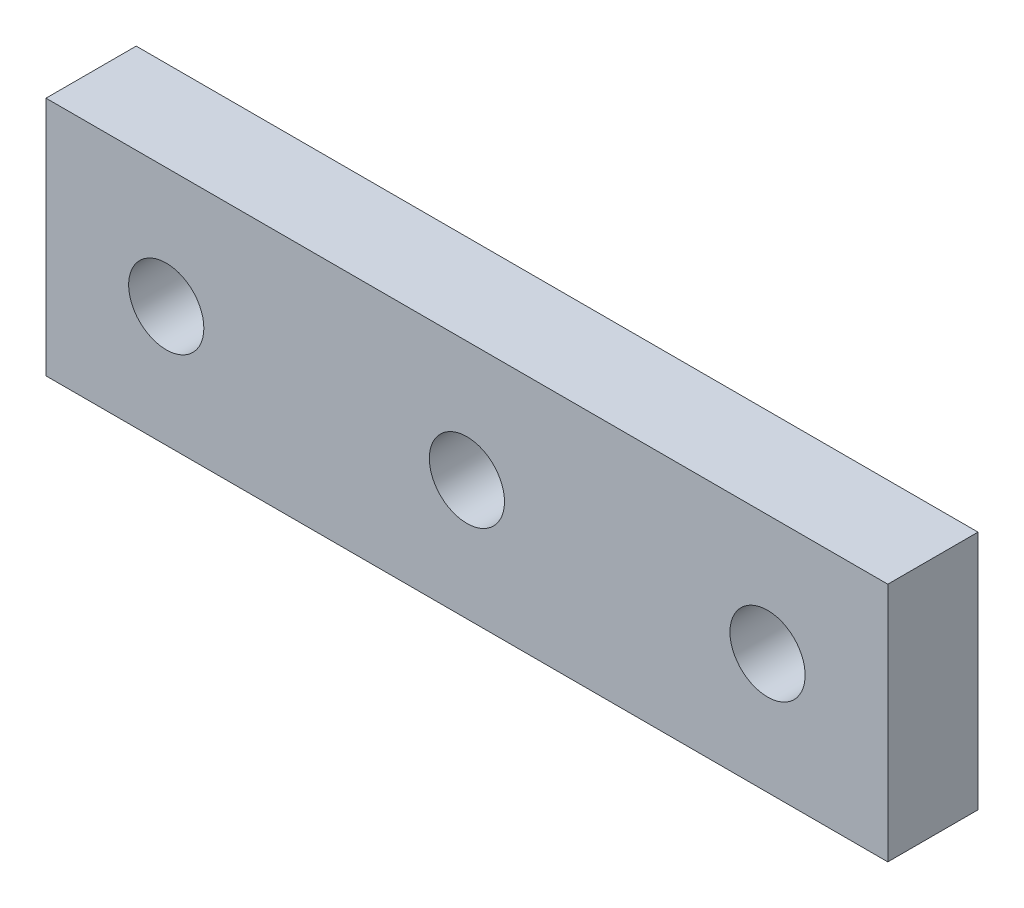
from build123d import *

# Parameters (mm, degrees)
SKETCH1_W             = 28
SKETCH1_H             = 8
SKETCH1_R             = 1.25
BOSS_EXTRUDE1_DEPTH   = 3
M3_TAPPED_HOLE6_D     = 2.5
M3_TAPPED_HOLE6_DEPTH = 7.5
M3_TAPPED_HOLE6_TIP   = 0.751075774
M3_TAPPED_HOLE1_D     = 2.5
M3_TAPPED_HOLE1_DEPTH = 7.5
M3_TAPPED_HOLE1_TIP   = 0.751075774


with BuildPart() as part:
    # Sketch1 → Boss-Extrude1 (new body)
    with BuildSketch(Plane.XY):
        with Locations((14, -4)):
            Rectangle(SKETCH1_W, SKETCH1_H)
        with Locations((4, -4)):
            Circle(SKETCH1_R, mode=Mode.SUBTRACT)
        with Locations(Location((24, -4, 0), (0, 0, 180))):
            Circle(SKETCH1_R, mode=Mode.SUBTRACT)
    extrude(amount=BOSS_EXTRUDE1_DEPTH)

    # M3 Tapped Hole6
    with Locations(Plane(origin=(4, -4, 3), x_dir=(1, 0, 0), z_dir=(0, 0, 1))):
        with Locations((0, 0), (20, 0)):
            Hole(M3_TAPPED_HOLE6_D / 2, depth=M3_TAPPED_HOLE6_DEPTH)
            with Locations((0, 0, -(M3_TAPPED_HOLE6_DEPTH + M3_TAPPED_HOLE6_TIP / 2))):  # 118° drill point
                Cone(0, M3_TAPPED_HOLE6_D / 2, M3_TAPPED_HOLE6_TIP, mode=Mode.SUBTRACT)

    # M3 Tapped Hole1
    with Locations(Plane(origin=(14, -4, 3), x_dir=(1, 0, 0), z_dir=(0, 0, 1))):
        with Locations((0, 0)):
            Hole(M3_TAPPED_HOLE1_D / 2, depth=M3_TAPPED_HOLE1_DEPTH)
            with Locations((0, 0, -(M3_TAPPED_HOLE1_DEPTH + M3_TAPPED_HOLE1_TIP / 2))):  # 118° drill point
                Cone(0, M3_TAPPED_HOLE1_D / 2, M3_TAPPED_HOLE1_TIP, mode=Mode.SUBTRACT)


solid = part.part
